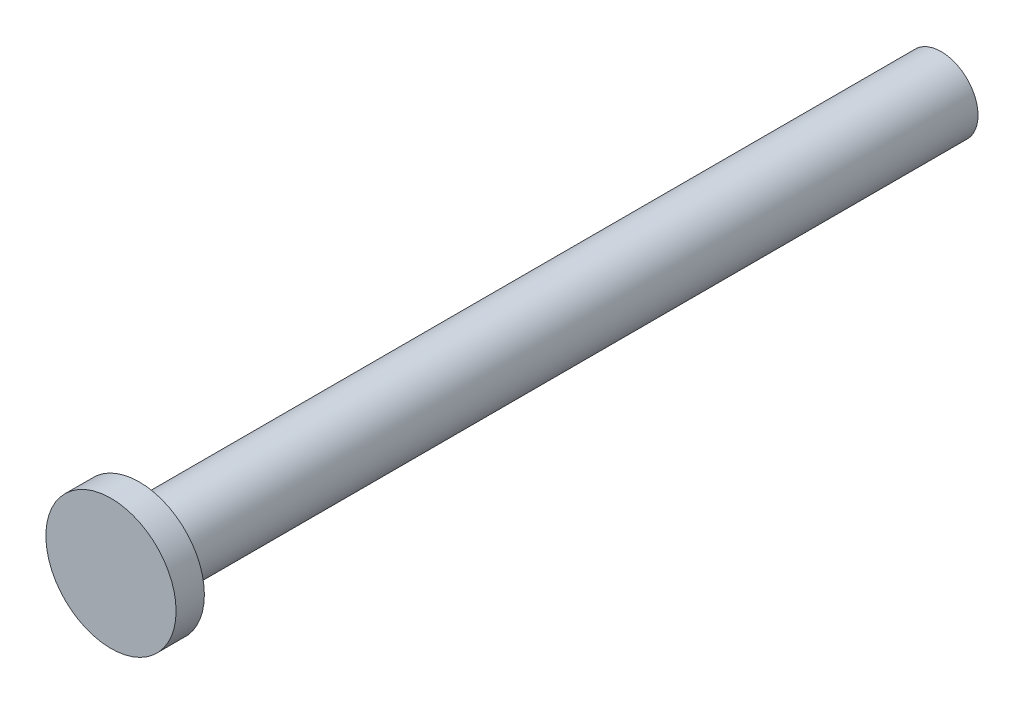
from build123d import *

# Parameters (mm, degrees)
BOSS_EXTRUDE1_DEPTH      = 38
BOSS_EXTRUDE1_DEPTH_BACK = 50
SKETCH1_R                = 3.9
SKETCH2_R                = 6.9
BOSS_EXTRUDE2_DEPTH      = 3


with BuildPart() as part:
    # Sketch1 → Boss-Extrude1 (new, two sides: drawn at the far end of the back side and taken through both)
    with BuildSketch(Plane.XY.offset(-BOSS_EXTRUDE1_DEPTH_BACK)):
        with Locations((-0.613489308, -35)):
            Circle(SKETCH1_R)
    extrude(amount=BOSS_EXTRUDE1_DEPTH + BOSS_EXTRUDE1_DEPTH_BACK)

    # Sketch2 → Boss-Extrude2 (add)
    with BuildSketch(Plane.XY.offset(38)):
        with Locations((-0.613489308, -35)):
            Circle(SKETCH2_R)
    extrude(amount=-BOSS_EXTRUDE2_DEPTH)


solid = part.part
